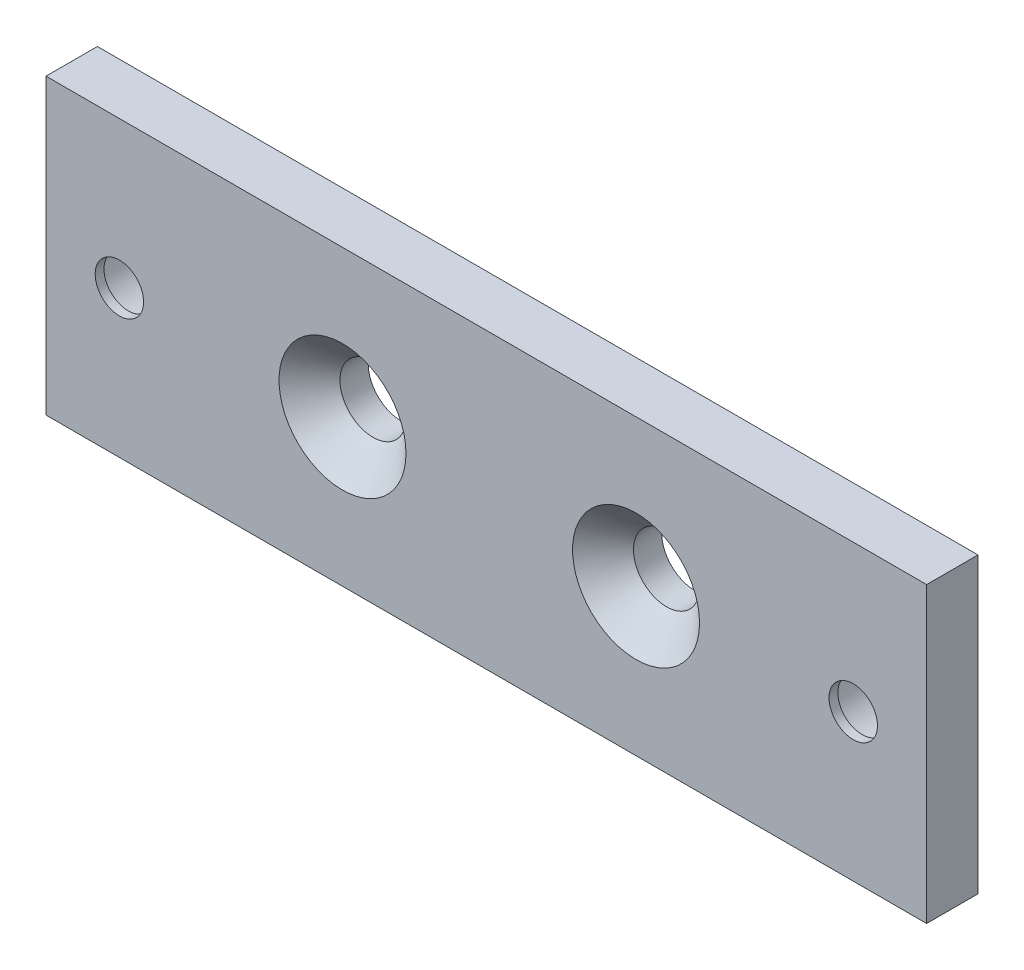
SolidWorks part; units mm, degrees
material "6061 合金"
ref_plane "前视基准面" through (0, 0, 0) normal (0, 0, 1) x (1, 0, 0)
ref_plane "上视基准面" through (0, 0, 0) normal (0, 1, 0) x (1, 0, 0)
ref_plane "右视基准面" through (0, 0, 0) normal (1, 0, 0) x (0, 0, -1)
sketch "草图1" plane through (0, 0, 0) normal (0, 0, 1) x (1, 0, 0)
  line L1 (-60, 20) -> (60, 20)
  line L2 (-60, 20) -> (-60, -20)
  line L3 (-60, -20) -> (60, -20)
  line L4 (60, 20) -> (60, -20)
  line L5 (-60, 20) -> (60, -20) construction
  line L6 (-60, -20) -> (60, 20) construction
  point P0 (0, 0)
  dimension "D1" = 120
  dimension "D2" = 40
extrude "凸台-拉伸1" add sketch "草图1" along normal mid plane 8
hole_wizard "打孔尺寸(%根据十字)槽沉头木螺钉的类型1" positions "3D草图1" profile "草图2" countersink size "M8" standard "GB"
sketch3d "3D草图1"
  line L0 (-60, -20, 4) -> (60, -20, 4) construction
  point P0 (-19.5959, 0, 4)
  point P2 (20.4041, 0, 4)
  dimension "D1" = 40
  dimension "D2" = 20
  dimension "D3" = 20
  dimension "D4" = 20
sketch "草图2" plane through (-19.5959, 0, 4) normal (1, 0, 0) x (0, -1, 0)
  line L0 (0, 0) -> (0, 12.7039)
  line L1 (0, 12.7039) -> (4.5, 10)
  line L2 (4.5, 10) -> (4.5, 4.15)
  line L3 (4.5, 4.15) -> (8.65, 0)
  line L5 (8.65, 0) -> (0, 0)
  line L6 (-4.5, 4.15) -> (-8.65, 0) construction
  line L10 (0, 12.7039) -> (-4.5, 10) construction
  line L11 (0, -6.35) -> (0, 107.95) construction
  dimension "孔直径" = 9
  dimension "孔深度" = 10
  dimension "近端锥形沉头孔直径" = 17.3
  dimension "近端锥形沉头孔角度" = 90
  dimension "导头角度" = 118
hole_wizard "打孔尺寸(%根据)内六角圆柱头螺钉的类型1" positions "3D草图2" profile "草图3" counterbore size "M6" standard "GB"
sketch3d "3D草图2"
  line L0 (-60, -20, -4) -> (60, -20, -4) construction
  line L1 (60, -20, -4) -> (60, 20, -4) construction
  line L2 (-60, 20, -4) -> (-60, -20, -4) construction
  point P0 (50, 0, -4)
  point P2 (-50, 0, -4)
  dimension "D1" = 20
  dimension "D2" = 20
  dimension "D3" = 10
  dimension "D4" = 10
sketch "草图3" plane through (50, 0, -4) normal (1, 0, 0) x (0, 1, 0)
  line L0 (0, 0) -> (0, 11.9828)
  line L1 (0, 11.9828) -> (3.3, 10)
  line L2 (3.3, 10) -> (3.3, 6.8)
  line L3 (3.3, 6.8) -> (5.5, 6.8)
  line L4 (5.5, 6.8) -> (5.5, 0)
  line L5 (5.5, 0) -> (0, 0)
  line L10 (0, 11.9828) -> (-3.3, 10) construction
  line L11 (0, -6.35) -> (0, 107.95) construction
  dimension "孔直径" = 6.6
  dimension "孔深度" = 10
  dimension "柱形沉头孔直径" = 11
  dimension "柱形沉头孔深度" = 6.8
  dimension "导头角度" = 118
chamfer "倒角1" distance 1 angle 45 4 edges at (60, 0, -4) (0, -20, -4) (0, 20, -4) (-60, 0, -4)
